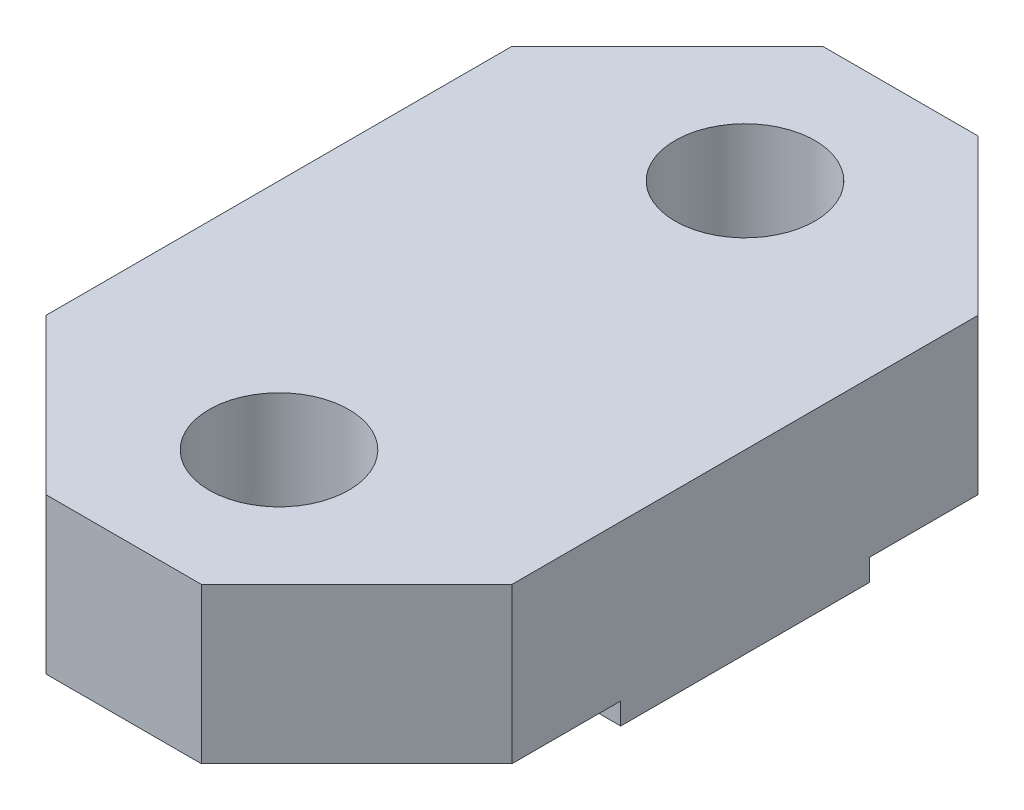
from build123d import *

# Parameters (mm, degrees)
SKETCH1_W                  = 15
SKETCH1_H                  = 25
BOSS_EXTRUDE1_DEPTH        = 5.7
SKETCH2_W                  = 15
SKETCH2_H                  = 8.5
CUT_EXTRUDE1_DEPTH         = 0.7
CHAMFER1_SIZE              = 5
F_4_5_4_5_DIAMETER_HOLE1_D = 4.5


with BuildPart() as part:
    # Sketch1 → Boss-Extrude1 (new body)
    with BuildSketch(Plane(origin=(0, 0, 0), x_dir=(1, 0, 0), z_dir=(0, 1, 0))):
        Rectangle(SKETCH1_W, SKETCH1_H)
    extrude(amount=BOSS_EXTRUDE1_DEPTH)

    # Sketch2 → Cut-Extrude1 (cut)
    with BuildSketch(Plane.XZ):
        with Locations((0, -8.25)):
            Rectangle(SKETCH2_W, SKETCH2_H)
        with Locations((0, 8.25)):
            Rectangle(SKETCH2_W, SKETCH2_H)
    extrude(amount=-CUT_EXTRUDE1_DEPTH, mode=Mode.SUBTRACT)

    # Chamfer1
    chamfer1_edges = [part.edges().sort_by_distance(p)[0] for p in [
        (7.5, 3.2, 12.5),
        (-7.5, 3.2, 12.5),
        (-7.5, 3.2, -12.5),
        (7.5, 3.2, -12.5),
    ]]
    chamfer(chamfer1_edges, length=CHAMFER1_SIZE)

    # Ø4.5 (4.5) Diameter Hole1 (through all)
    with Locations(Plane(origin=(0, 5.7, 0), x_dir=(1, 0, 0), z_dir=(0, 1, 0))):
        with Locations((0, 7.5), (0, -7.5)):
            Hole(F_4_5_4_5_DIAMETER_HOLE1_D / 2)


solid = part.part
